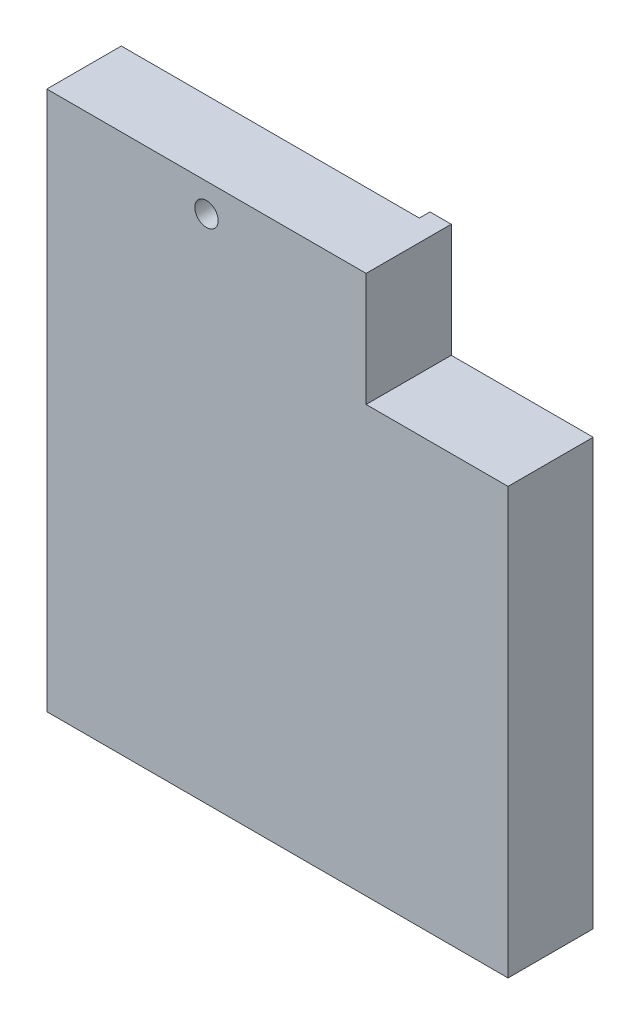
from build123d import *

# Parameters (mm, degrees)
SKETCH_1_W          = 65
SKETCH_1_H          = 60
EXTRUDE_1_DEPTH     = 12
SKETCH_4_W          = 45
SKETCH_4_H          = 16
EXTRUDE_2_DEPTH     = 12
SKETCH_5_W          = 42
SKETCH_5_H          = 76
CUT_EXTRUDE_1_DEPTH = 1.5
HOLE_WIZARD_M4_1_D  = 3.3


with BuildPart() as part:
    # 草图1 → 凸台-拉伸1 (new body)
    with BuildSketch(Plane.XY):
        Rectangle(SKETCH_1_W, SKETCH_1_H)
    extrude(amount=EXTRUDE_1_DEPTH)

    # 草图4 → 凸台-拉伸2 (add)
    with BuildSketch(Plane(origin=(0, 0, 0), x_dir=(-1, 0, 0), z_dir=(0, 0, -1))):
        with Locations((10, 38)):
            Rectangle(SKETCH_4_W, SKETCH_4_H)
    extrude(amount=-EXTRUDE_2_DEPTH)

    # 草图5 → 切除-拉伸1 (cut)
    with BuildSketch(Plane(origin=(0, 0, 0), x_dir=(-1, 0, 0), z_dir=(0, 0, -1))):
        with Locations((11.5, 8)):
            Rectangle(SKETCH_5_W, SKETCH_5_H)
    extrude(amount=-CUT_EXTRUDE_1_DEPTH, mode=Mode.SUBTRACT)

    # M4 螺纹孔1 (through all)
    with Locations(Plane(origin=(-10, 42, 12), x_dir=(1, 0, 0), z_dir=(0, 0, 1))):
        with Locations((0, 0)):
            Hole(HOLE_WIZARD_M4_1_D / 2)


solid = part.part
